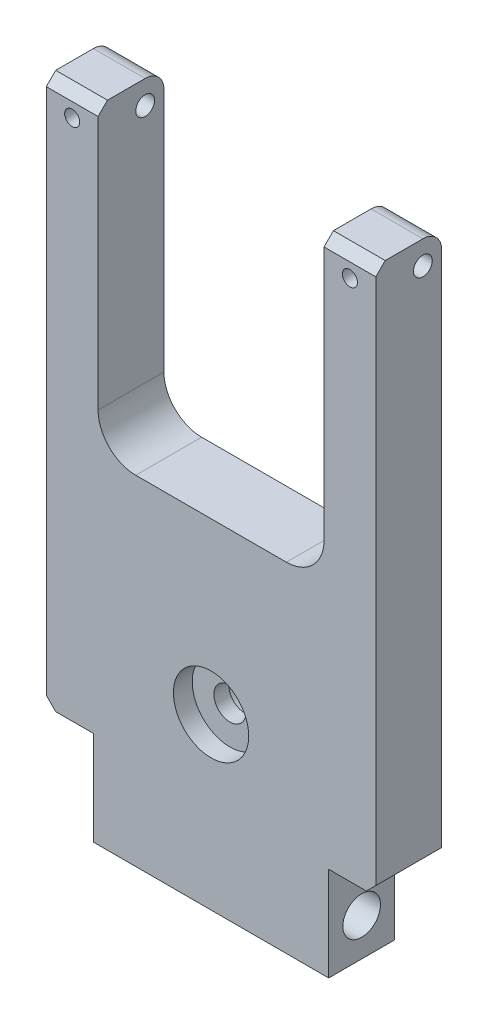
from build123d import *

# Parameters (mm, degrees)
BOSS_EXTRUDE1_DEPTH                                 = 7
SKETCH2_R                                           = 1
CUT_EXTRUDE1_DEPTH                                  = 77.798437484
SKETCH3_W                                           = 5
SKETCH3_H                                           = 10
CUT_EXTRUDE2_DEPTH                                  = 71.563800918
SKETCH4_R                                           = 2
CUT_EXTRUDE3_DEPTH                                  = 75.652528423
M3_TAPPED_HOLE1_REACH                               = 72.564
M3_TAPPED_HOLE1_BORE_R                              = 1.25
FILLET1_R                                           = 4
CHAMFER1_SIZE                                       = 1
SKETCH8_R                                           = 4
CUT_EXTRUDE4_DEPTH                                  = 2
FILLET2_R                                           = 2
M2_TAPPED_HOLE1_D                                   = 1.6
M2_TAPPED_HOLE1_DEPTH                               = 5.2
M2_TAPPED_HOLE1_TIP                                 = 0.480688495
CBORE_FOR_M3_HEX_SOCKET_HEAD_CAP_SCREW1_D           = 3.4
CBORE_FOR_M3_HEX_SOCKET_HEAD_CAP_SCREW1_CBORE_D     = 6.5
CBORE_FOR_M3_HEX_SOCKET_HEAD_CAP_SCREW1_CBORE_DEPTH = 3.4


with BuildPart() as part:
    # Sketch1 → Boss-Extrude1 (new body)
    with BuildSketch(Plane.XY):
        Polygon((17.5, 0), (-17.5, 0), (-17.5, 68), (-12, 68), (-12, 36), (12, 36), (12, 68), (17.5, 68), align=None)
    extrude(amount=BOSS_EXTRUDE1_DEPTH)

    # Sketch2 → Cut-Extrude1 (cut, through all)
    with BuildSketch(Plane(origin=(17.5, 0, 0), x_dir=(0, 0, -1), z_dir=(1, 0, 0))):
        with Locations((-2, 65.5)):
            Circle(SKETCH2_R)
    extrude(amount=-CUT_EXTRUDE1_DEPTH, mode=Mode.SUBTRACT)

    # Sketch3 → Cut-Extrude2 (cut, through all)
    with BuildSketch(Plane.XY.offset(7)):
        with Locations((-15, 5)):
            Rectangle(SKETCH3_W, SKETCH3_H)
        with Locations((15, 5)):
            Rectangle(SKETCH3_W, SKETCH3_H)
    extrude(amount=-CUT_EXTRUDE2_DEPTH, mode=Mode.SUBTRACT)

    # Sketch4 → Cut-Extrude3 (cut, through all)
    with BuildSketch(Plane(origin=(12.5, 0, 0), x_dir=(0, 0, -1), z_dir=(1, 0, 0))):
        with Locations((-3.5, 4)):
            Circle(SKETCH4_R)
    extrude(amount=-CUT_EXTRUDE3_DEPTH, mode=Mode.SUBTRACT)

    # M3 Tapped Hole1 bore → M3 Tapped Hole1 (cut, up to next)
    with BuildSketch(Plane.XZ, mode=Mode.PRIVATE) as m3_tapped_hole1_sk1:
        with Locations((7.5, 3.5)):
            Circle(M3_TAPPED_HOLE1_BORE_R)
    m3_tapped_hole1_tool1 = extrude(m3_tapped_hole1_sk1.sketch, amount=-M3_TAPPED_HOLE1_REACH, mode=Mode.PRIVATE) & part.part
    # M3 Tapped Hole1 bore → M3 Tapped Hole1 (cut, up to next)
    with BuildSketch(Plane.XZ, mode=Mode.PRIVATE) as m3_tapped_hole1_sk2:
        with Locations((-7.5, 3.5)):
            Circle(M3_TAPPED_HOLE1_BORE_R)
    m3_tapped_hole1_tool2 = extrude(m3_tapped_hole1_sk2.sketch, amount=-M3_TAPPED_HOLE1_REACH, mode=Mode.PRIVATE) & part.part
    add(m3_tapped_hole1_tool1.solids().sort_by_distance((7.5, 0, 3.5))[0], mode=Mode.SUBTRACT)
    add(m3_tapped_hole1_tool2.solids().sort_by_distance((-7.5, 0, 3.5))[0], mode=Mode.SUBTRACT)

    # Fillet1
    fillet1_edges = [part.edges().sort_by_distance(p)[0] for p in [
        (-12, 36, 3.5),
        (12, 36, 3.5),
    ]]
    fillet(fillet1_edges, radius=FILLET1_R)

    # Chamfer1
    chamfer1_edges = [part.edges().sort_by_distance(p)[0] for p in [
        (14.75, 68, 7),
        (-14.75, 68, 7),
        (-17.5, 10, 3.5),
        (17.5, 10, 3.5),
    ]]
    chamfer(chamfer1_edges, length=CHAMFER1_SIZE)

    # Sketch8 → Cut-Extrude4 (cut)
    with BuildSketch(Plane.XY.offset(7)):
        with Locations((0, 18)):
            Circle(SKETCH8_R)
    extrude(amount=-CUT_EXTRUDE4_DEPTH, mode=Mode.SUBTRACT)

    # Fillet2
    fillet2_edges = [part.edges().sort_by_distance(p)[0] for p in [
        (-14.75, 68, 0),
        (14.75, 68, 0),
    ]]
    fillet(fillet2_edges, radius=FILLET2_R)

    # M2 Tapped Hole1
    with Locations(Plane.XY.offset(7)):
        with Locations((-14.75, 65.5), (14.75, 65.5)):
            Hole(M2_TAPPED_HOLE1_D / 2, depth=M2_TAPPED_HOLE1_DEPTH)
            with Locations((0, 0, -(M2_TAPPED_HOLE1_DEPTH + M2_TAPPED_HOLE1_TIP / 2))):  # 118° drill point
                Cone(0, M2_TAPPED_HOLE1_D / 2, M2_TAPPED_HOLE1_TIP, mode=Mode.SUBTRACT)

    # CBORE for M3 Hex Socket Head Cap Screw1 (through all)
    with Locations(Plane(origin=(0, 0, 0), x_dir=(-1, 0, 0), z_dir=(0, 0, -1))):
        with Locations((0, 18)):
            CounterBoreHole(CBORE_FOR_M3_HEX_SOCKET_HEAD_CAP_SCREW1_D / 2, CBORE_FOR_M3_HEX_SOCKET_HEAD_CAP_SCREW1_CBORE_D / 2, CBORE_FOR_M3_HEX_SOCKET_HEAD_CAP_SCREW1_CBORE_DEPTH)


solid = part.part
